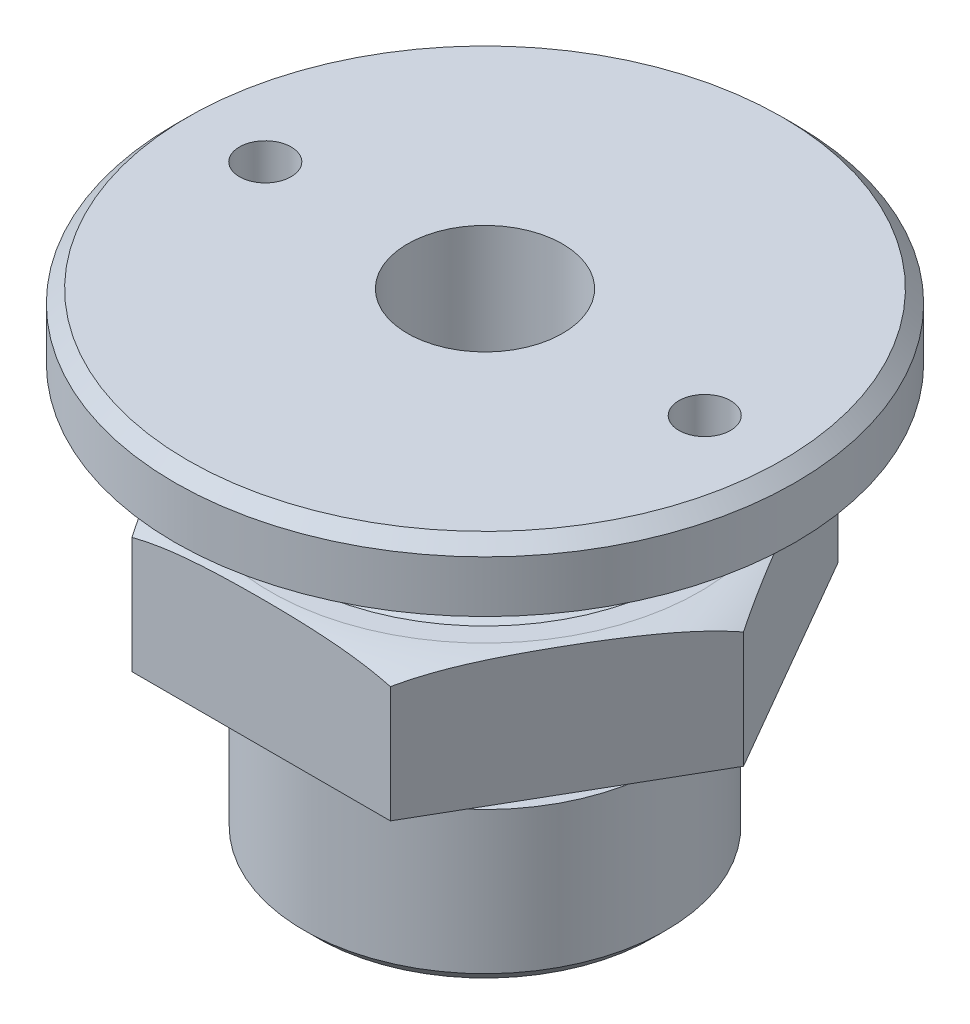
from build123d import *

# Parameters (mm, degrees)
CHAMFER2_SIZE      = 1
CUT_EXTRUDE1_START = -10
SKETCH2_R          = 31.378818645
CUT_EXTRUDE1_DEPTH = 10
CHAMFER3_SIZE      = 1
CUT_EXTRUDE2_REACH = 52.21
SKETCH4_R          = 2
SCALE_1_SCALE      = 1.875


with BuildPart() as part:
    # Sketch1 → Revolve2 (revolve)
    with BuildSketch(Plane.XY, mode=Mode.PRIVATE) as revolve2_sk:
        with BuildLine():
            Line((6, 0), (6, 37))
            Line((6, 37), (24, 37))
            Line((24, 37), (24, 32))
            Line((24, 32), (14, 32))
            ThreePointArc((14, 32), (12.392227943, 28.198889706), (15, 25))
            Line((15, 25), (20, 25))
            Line((20, 25), (20, 15))
            Line((20, 15), (10, 15))
            Line((10, 15), (10, 12))
            Line((10, 12), (14, 12))
            Line((14, 12), (14, 0))
            Line((14, 0), (6, 0))
        make_face()
    revolve(revolve2_sk.sketch.rotate(Axis((0, 0, 0), (0, 1, 0)), 90), axis=Axis((0, 0, 0), (0, 1, 0)))

    # Chamfer2
    chamfer2_edges = [part.edges().sort_by_distance(p)[0] for p in [
        (0, 0, 14),
    ]]
    chamfer(chamfer2_edges, length=CHAMFER2_SIZE)

    # Sketch2 → Cut-Extrude1 (cut)
    with BuildSketch(Plane(origin=(0, 25, 0), x_dir=(1, 0, 0), z_dir=(0, 1, 0)).offset(CUT_EXTRUDE1_START)):
        Circle(SKETCH2_R)
        Polygon((20, 0), (10, 17.320508076), (-10, 17.320508076), (-20, 0), (-10, -17.320508076), (10, -17.320508076), align=None, mode=Mode.SUBTRACT)
    extrude(amount=CUT_EXTRUDE1_DEPTH, mode=Mode.SUBTRACT)

    # Sketch3 → Cut-Revolve1 (revolve, cut)
    with BuildSketch(Plane.XY, mode=Mode.PRIVATE) as cut_revolve1_sk:
        with BuildLine():
            Line((-20, 24), (-20, 25))
            Line((-20, 25), (-16.614510602, 25))
            ThreePointArc((-16.614510602, 25), (-18.356765058, 24.667614757), (-20, 24))
        make_face()
    revolve(cut_revolve1_sk.sketch.rotate(Axis((0, 0, 0), (0, 1, 0)), 270), axis=Axis((0, 0, 0), (0, 1, 0)), mode=Mode.SUBTRACT)

    # Chamfer3
    chamfer3_edges = [part.edges().sort_by_distance(p)[0] for p in [
        (0, 37, 24),
    ]]
    chamfer(chamfer3_edges, length=CHAMFER3_SIZE)

    # Sketch4 → Cut-Extrude2 (cut, up to next)
    with BuildSketch(Plane(origin=(0, 37, 0), x_dir=(1, 0, 0), z_dir=(0, 1, 0)), mode=Mode.PRIVATE) as cut_extrude2_sk1:
        with Locations(Location((17, 0, 0), (0, 0, 270))):
            Circle(SKETCH4_R)
    cut_extrude2_tool1 = extrude(cut_extrude2_sk1.sketch, amount=-CUT_EXTRUDE2_REACH, mode=Mode.PRIVATE) & part.part
    # Sketch4 → Cut-Extrude2 (cut, up to next)
    with BuildSketch(Plane(origin=(0, 37, 0), x_dir=(1, 0, 0), z_dir=(0, 1, 0)), mode=Mode.PRIVATE) as cut_extrude2_sk2:
        with Locations(Location((-17, 0, 0), (0, 0, 90))):
            Circle(SKETCH4_R)
    cut_extrude2_tool2 = extrude(cut_extrude2_sk2.sketch, amount=-CUT_EXTRUDE2_REACH, mode=Mode.PRIVATE) & part.part
    add(cut_extrude2_tool1.solids().sort_by_distance((17, 37, 0))[0], mode=Mode.SUBTRACT)
    add(cut_extrude2_tool2.solids().sort_by_distance((-17, 37, 0))[0], mode=Mode.SUBTRACT)


with BuildPart() as part_1:
    # Scale 1: scaled about (-3.12e-07, 22.102096906, 1.9e-08)
    add(part.part.scale(SCALE_1_SCALE).moved(Location((2.73e-07, -19.339334793, -1.7e-08))))


solid = part_1.part
